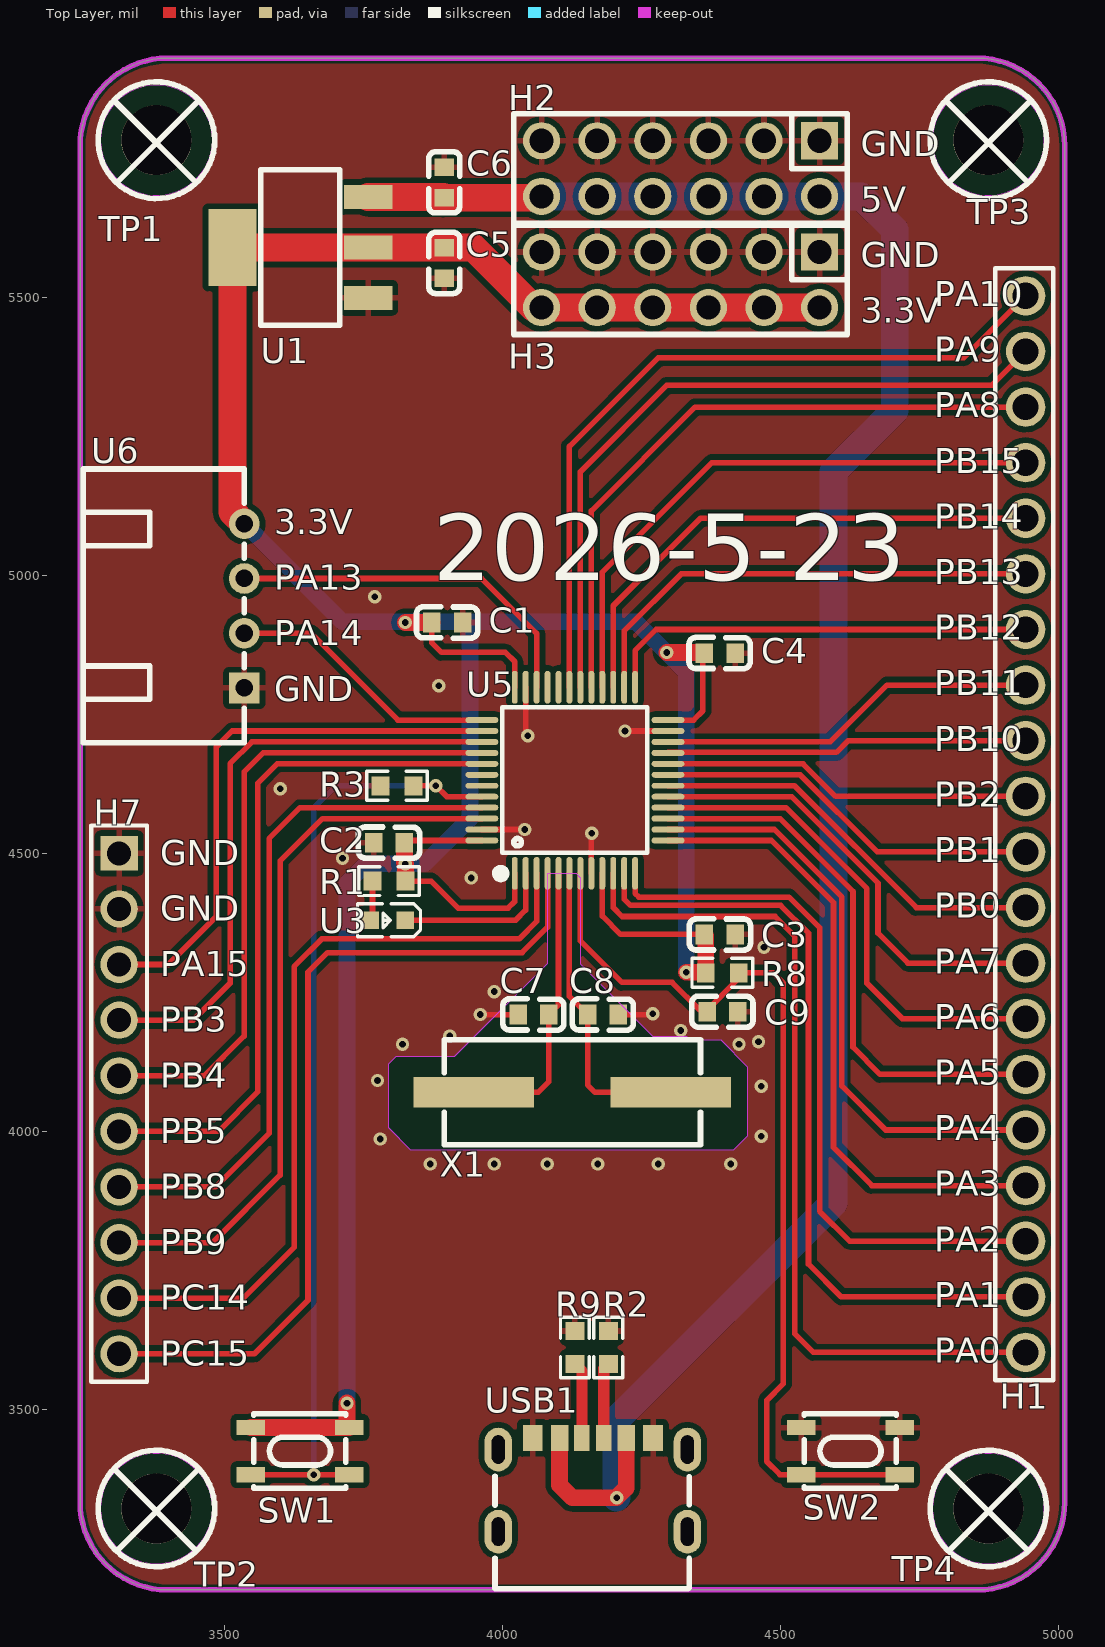
[diagram p0: Top Layer view]
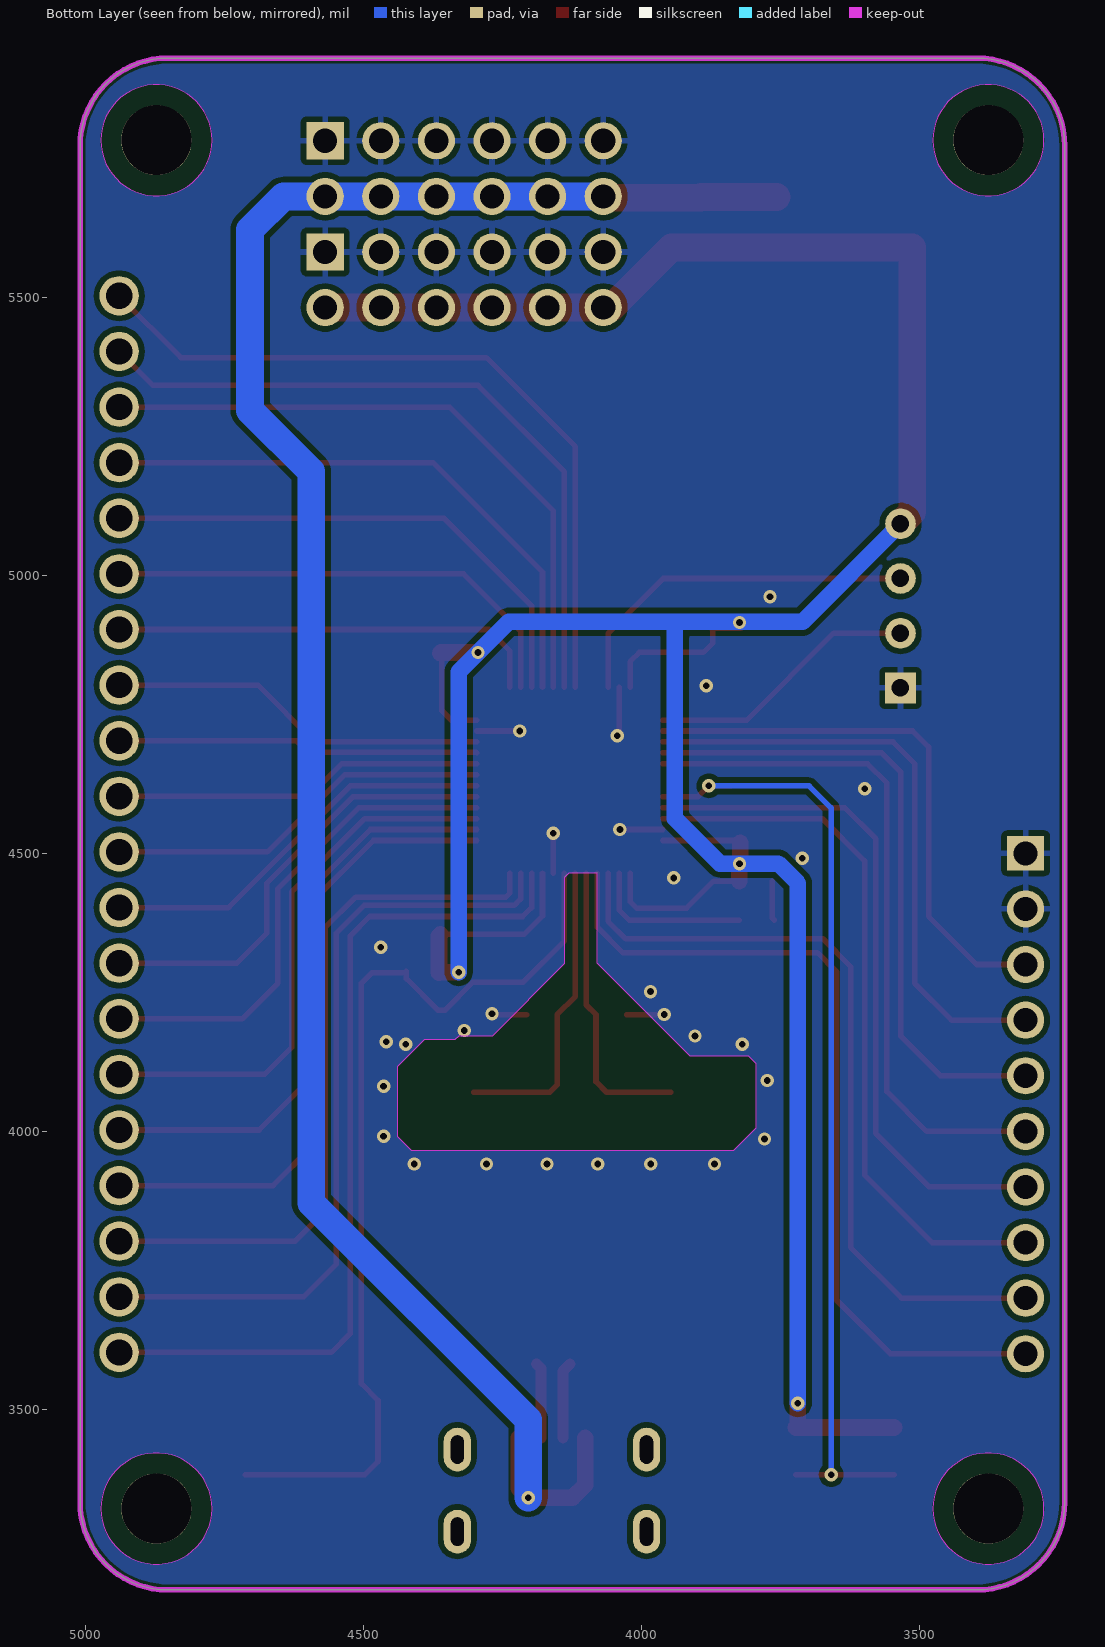
[diagram p1: Bottom Layer view, seen from below]
# Altium PCB MISC89146.pcbdoc
Units mil, origin at the board's own origin, x right, y up, seen from the top; angles counter-clockwise.
Board outline 1770.59 x 2754.61 mil, 2 copper layers (Top Layer, Bottom Layer), stack 62.206 mil thick; 30 components, 45 nets, 164 pads, 36 vias.

## Layer stack, top to bottom
Top Solder Mask Layer: solder mask 0.394, Dk 3.3
Top Layer: signal copper 1.379
Dielectric1: surface 59.449, FR4, Dk 4.5
Bottom Layer: signal copper 1.378
Bottom Solder Mask Layer: solder mask 0.394, Dk 3.3

## Board outline
3397.18,5930 ccw(c3397.18,5772.52) 3239.7,5772.52 3239.7,3332.87 ccw(c3397.18,3332.87) 3397.18,3175.39 4852.81,3175.39 ccw(c4852.81,3332.87) 5010.3,3332.87 5010.3,5772.52 ccw(c4852.81,5772.52) 4852.81,5930 3397.18,5930

## Design rules (kind name [scope] priority, off if disabled: settings)
BoardOutlineClearance copperThickness2oz_1 [All] p2 off: genericclearance=7.99 ignorepadtopadclearanceinfootprint=FALSE except(0: Arc-SplitContinuation Track-SplitContinuation SMDPad-SplitContinuation THPad-SplitContinuation Via-SplitContinuation Fill-SplitContinuation Region-SplitContinuation Poly-SplitContinuation Text-SplitContinuation Hole-SplitContinuation; 5.98: Arc-CutoutEdge SMDPad-CutoutEdge THPad-CutoutEdge Via-CutoutEdge Fill-CutoutEdge Region-CutoutEdge Text-CutoutEdge; 6.93: Hole-OutlineEdge Hole-CutoutEdge; 10: Poly-OutlineEdge Poly-CutoutEdge; 11.81: Arc-OutlineEdge Track-OutlineEdge SMDPad-OutlineEdge THPad-OutlineEdge Via-OutlineEdge Fill-OutlineEdge Region-OutlineEdge Text-OutlineEdge Track-CutoutEdge)
BoardOutlineClearance copperThickness1oz_1 [All] p4: genericclearance=4.02 ignorepadtopadclearanceinfootprint=FALSE except(0: Arc-SplitContinuation Track-SplitContinuation SMDPad-SplitContinuation THPad-SplitContinuation Via-SplitContinuation Fill-SplitContinuation Region-SplitContinuation Poly-SplitContinuation Text-SplitContinuation Hole-SplitContinuation; 6: SMDPad-CutoutEdge THPad-CutoutEdge Via-CutoutEdge Fill-CutoutEdge Region-CutoutEdge Text-CutoutEdge; 6.93: Hole-OutlineEdge Hole-CutoutEdge; 10: Poly-OutlineEdge Poly-CutoutEdge; 11.8: Arc-OutlineEdge Track-OutlineEdge SMDPad-OutlineEdge THPad-OutlineEdge Via-OutlineEdge Fill-OutlineEdge Region-OutlineEdge Text-OutlineEdge; 11.81: Arc-CutoutEdge Track-CutoutEdge)
Clearance copperThickness2oz [All] p1 off: gap=7.99 ignorepadtopadclearanceinfootprint=FALSE except(5.98: SMDPad-Track SMDPad-SMDPad THPad-Track SMDPad-THPad THPad-THPad Track-Via SMDPad-Via THPad-Via Via-Via Fill-Track Region-Track Fill-SMDPad Region-SMDPad Fill-THPad Region-THPad Fill-Via Region-Via Fill-Fill Fill-Region Region-Region Arc-Track Arc-SMDPad Arc-THPad Arc-Via Fill-Arc Region-Arc Arc-Arc Text-Track SMDPad-Text Text-THPad Text-Via Fill-Text Region-Text Arc-Text Text-Text; 6.93: Hole-Track Hole-SMDPad Hole-THPad Hole-Via Fill-Hole Region-Hole Hole-Arc Hole-Text; 10: Poly-Track Poly-SMDPad Poly-THPad Poly-Via Poly-Fill Poly-Region Poly-Poly Poly-Arc Poly-Text Poly-Hole)
Clearance copperThickness1oz [All] p3: gap=4.02 ignorepadtopadclearanceinfootprint=FALSE except(5.98: SMDPad-Track SMDPad-SMDPad THPad-Track SMDPad-THPad THPad-THPad Track-Via SMDPad-Via THPad-Via Via-Via Fill-Track Region-Track Fill-SMDPad Region-SMDPad Fill-THPad Region-THPad Fill-Via Region-Via Fill-Fill Fill-Region Region-Region; 6: Arc-Track Arc-SMDPad Arc-THPad Arc-Via Fill-Arc Region-Arc Arc-Arc Text-Track SMDPad-Text Text-THPad Text-Via Fill-Text Region-Text Arc-Text Text-Text; 6.93: Hole-Track Hole-SMDPad Hole-THPad Hole-Via Fill-Hole Region-Hole Hole-Arc Hole-Text; 10: Poly-Track Poly-SMDPad Poly-THPad Poly-Via Poly-Fill Poly-Region Poly-Poly Poly-Arc Poly-Text Poly-Hole)
Creepage creepage [All] p1: checkdistance=0 ignoreinternallayers=TRUE applytopolygonpour=TRUE
DiffPairsRouting differentialPair [All] p1: maxlimit=6 minlimit=6 mostfreqgap=6 toplayer_minwidth=5 toplayer_prefwidth=10 toplayer_maxwidth=100 toplayer_mingap=6 toplayer_prefgap=6 toplayer_maxgap=6 bottomlayer_minwidth=5 bottomlayer_prefwidth=10 bottomlayer_maxwidth=100 bottomlayer_mingap=6 bottomlayer_prefgap=6 bottomlayer_maxgap=6 maxuncoupledlength=10
HoleToHoleClearance otherClearance [All] p1: gap=11.81 allowstackedmicrovias=TRUE
Length netLength [All] p1: minlimit=0 maxlimit=0
MatchedLengths netLengthTolerance [All] p1: tolerance=1000
PasteMaskExpansion pasteMaskExpansion [All] p1: expansion=0
PlaneConnect innerPlane [All] p1: planeconnectstyle=Relief reliefexpansion=20 reliefentries=4 reliefconductorwidth=10 reliefairgap=10
PolygonConnect copperRegion [(InNet('GND'))] p1: connectstyle=Relief reliefconductorwidth=10 reliefentries=4 polygonreliefangle="90 Angle" airgapwidth=10 via.connectstyle=Relief via.reliefconductorwidth=10 via.reliefentries=4 via.polygonreliefangle="90 Angle" via.airgapwidth=10
RoutingVias viaSize [All] p1: holewidth=12.01 width=24.02 viastyle="Through Hole" minholewidth=11.81 minwidth=19.68 maxholewidth=248.03 maxwidth=393.7
SolderMaskExpansion solderMaskExpansion [IsVia] p1: expansion=-1000 istentingtop=TRUE
SolderMaskExpansion solderMaskExpansion [All] p2: expansion=2 istentingtop=FALSE
Width copperThickness2oz_2 [All] p1 off: maxlimit=100 minlimit=8 preferedwidth=10
Width copperThickness1oz_2 [All] p2: maxlimit=100 minlimit=5 preferedwidth=10

## Components (designator, comment, footprint, x,y, rotation, side; value= is the part's Value field where it differs from the comment)
C1 "100nF" C0603 3900,4915 r0 top
C2 "100nF" C0603 3795.45,4519.09 r0 top
C3 "100nF" C0603 4390,4354.09 r180 top
C4 "100nF" C0603 4390,4860 r0 top
C5 "2.2UF" C0603 3894.56,5561.33 r270 top
C6 "10UF" C0603 3894.56,5706.33 r270 top
C7 "22PF" C0603 4055,4210 r0 top
C8 "22PF" C0603 4180,4210 r0 top
C9 "1UF" C0603 4395,4215 r0 top
H1 "" HDR-TH_20P-P2.54-V-M-1 4940,4552.46 r90 top
H2 "" HDR-TH_12P-P2.54-V-M-R2-C6-S2.54 4319.56,5731.33 r180 top
H3 "" HDR-TH_12P-P2.54-V-M-R2-C6-S2.54 4319.56,5531.33 r180 top
H7 "" hdr-th_10p-p2.54-v-m-1 3310,4050 r270 top
R1 "1K" R0603 3795.15,4450 r180 top
R2 "5K1" R0603 4189.56,3611.33 r270 top
R3 "10K" R0603 3809.56,4621.33 r0 top
R8 "10K" R0603 4394.69,4285 r0 top
R9 "5K1" R0603 4129.56,3611.33 r270 top
SW1 "TS-KG89S-AT25F" SW-SMD_4P-L4.2-W3.3-P2.15-LS5.1 3635,3425 r180 top
SW2 "TS-KG89S-AT25F" SW-SMD_4P-L4.2-W3.3-P2.15-LS5.1 4625,3425 r180 top
TP1 "" M3 3376.97,5782.36 r0 top
TP2 "" M3 3376.97,3321.65 r0 top
TP3 "" M3 4873.03,5782.36 r0 top
TP4 "" M3 4873.03,3321.65 r0 top
U1 "" SOT_223 3634.7,5589.36 r90 top
U3 "LED_0603" LED_0603 3791.2,4379.5 r180 top
U5 "CH32V203C8T6" LQFP-48_L7.0-W7.0-P0.50-LS9.0-BL 4129.56,4631.33 r0 top
U6 "HCZZ0139-4" CONN-TH_4P-P2.50_HCZZ0139-4 3535,4945 r270 top
USB1 "" "USB_ TYPE-C-6P" 4156.74,3364.36 r0 top
X1 "8M-HC-49SMD" CRYSTAL-SMD_L11.4-W4.7-LS12.7 4125,4070 r180 top

## Footprints (in the part's own frame and the unit in brackets; to place one, negate y for a bottom-side part, rotate by r counter-clockwise, add the part's x,y. Pads: shape width x height; smd on the part's side, far side on the other; paste and mask are expansions set on the pad)
C0603 [mm]
  rect 0.8x0.9 smd paste+0 mask+0.051: 1(-0.7,0) 2(0.7,0)
  silkscreen extent -1.41,-0.71 1.39,0.72
CONN-TH_4P-P2.50_HCZZ0139-4 [mm]
  round 1.4 hole 0.8: 1(-3.75,0) 2(-1.25,0) 3(1.25,0)
  rect 1.4x1.4 hole 0.8: 4(3.75,0)
  silkscreen extent -6.25,-7.37 6.25,0
CRYSTAL-SMD_L11.4-W4.7-LS12.7 [mm]
  rect 5.5x1.4 smd paste+0 mask+0.051: 1(-4.5,0) 2(4.5,0)
  silkscreen extent -5.85,-2.4 5.85,2.4
hdr-th_10p-p2.54-v-m-1 [mm]
  rect 1.575x1.7 hole 1.1: 1(-11.43,0)
  round 1.7 hole 1.1: 2(-8.89,0) 3(-6.35,0) 4(-3.81,0) 5(-1.27,0) 6(1.27,0) 7(3.81,0) 8(6.35,0) 9(8.89,0) 10(11.43,0)
  silkscreen extent -12.7,-1.27 12.7,1.27
HDR-TH_12P-P2.54-V-M-R2-C6-S2.54 [mm]
  rect 1.7x1.7 hole 1.1: 1(-6.35,-1.27)
  round 1.7 hole 1.1: 2(-6.35,1.27) 3(-3.81,-1.27) 4(-3.81,1.27) 5(-1.27,-1.27) 6(-1.27,1.27) 7(1.27,-1.27) 8(1.27,1.27) 9(3.81,-1.27) 10(3.81,1.27) 11(6.35,-1.27) 12(6.35,1.27)
  silkscreen extent -7.62,-2.5 7.62,2.5
HDR-TH_20P-P2.54-V-M-1 [mm]
  round 1.8 hole 1.2 paste+0 mask+0.051: 1(-24.13,0) 2(-21.59,0) 3(-19.05,0) 4(-16.51,0) 5(-13.97,0) 6(-11.43,0) 7(-8.89,0) 8(-6.35,0) 9(-3.81,0) 10(-1.27,0) 11(1.27,0) 12(3.81,0) 13(6.35,0) 14(8.89,0) 15(11.43,0) 16(13.97,0) 17(16.51,0) 18(19.05,0) 19(21.59,0) 20(24.13,0)
  silkscreen extent -25.4,-1.27 25.4,1.4
LED_0603 [mil]
  rect 31.5x31.5 smd paste+0 mask+2: 1(-33.5,-0.4) 2(29.5,-0.2)
  silkscreen extent -61,-30 53,30
LQFP-48_L7.0-W7.0-P0.50-LS9.0-BL [mm]
  oval 0.27x1.5 smd paste+0 mask+0.05: 1(-2.75,-4.25) 2(-2.25,-4.25) 3(-1.75,-4.25) 4(-1.25,-4.25) 5(-0.75,-4.25) 6(-0.25,-4.25) 7(0.25,-4.25) 8(0.75,-4.25) 9(1.25,-4.25) 10(1.75,-4.25) 11(2.25,-4.25) 12(2.75,-4.25) 25(2.75,4.25) 26(2.25,4.25) 27(1.75,4.25) 28(1.25,4.25) 29(0.75,4.25) 30(0.25,4.25) 31(-0.25,4.25) 32(-0.75,4.25) 33(-1.25,4.25) 34(-1.75,4.25) 35(-2.25,4.25) 36(-2.75,4.25)
  oval 1.5x0.27 smd paste+0 mask+0.05: 13(4.25,-2.75) 14(4.25,-2.25) 15(4.25,-1.75) 16(4.25,-1.25) 17(4.25,-0.75) 18(4.25,-0.25) 19(4.25,0.25) 20(4.25,0.75) 21(4.25,1.25) 22(4.25,1.75) 23(4.25,2.25) 24(4.25,2.75) 37(-4.25,2.75) 38(-4.25,2.25) 39(-4.25,1.75) 40(-4.25,1.25) 41(-4.25,0.75) 42(-4.25,0.25) 43(-4.25,-0.25) 44(-4.25,-0.75) 45(-4.25,-1.25) 46(-4.25,-1.75) 47(-4.25,-2.25) 48(-4.25,-2.75)
  silkscreen extent -3.59,-4.46 3.3,3.34
M3 [mil]
  round 126 hole 126 paste+0 mask+4: 0(0,0)
  Board Outline Layer region: 100,0 90.1,-43.39 62.35,-78.18 22.25,-97.49 -22.25,-97.49 -62.35,-78.18 -90.1,-43.39 -100,0 -100,0 -90.1,43.39 -62.35,78.18 -22.25,97.49 22.25,97.49 62.35,78.18 90.1,43.39 100,0
  silkscreen extent -105,-105 105,105
R0603 [mil]
  rect 31.75x34.02 smd paste-3937.01 mask+2: 1(-29.66,0) 2(29.66,0)
  silkscreen extent -55,-26 55,26
SOT_223 [mil]
  rect 43.3x86.6 smd paste+0 mask+2: 1(-90.5,-123.05) 2(0,-123.05) 3(90.6,-123.05)
  rect 137.8x86.6 smd paste+0 mask+2: 4(0,120.95)
  silkscreen extent -140,-72 140,70
SW-SMD_4P-L4.2-W3.3-P2.15-LS5.1 [mm]
  rect 1.3x0.7 smd paste+0 mask+0.051: 1(-2.25,1.075) 2(2.25,1.075) 3(-2.25,-1.075) 4(2.25,-1.075)
  silkscreen extent -2.1,-1.7 2.1,1.7
"USB_ TYPE-C-6P" [mm]
  oval 1.25x2 hole 0.6 slot 1.3 at 90 deg paste+0 mask+0.05: 7(-4.193,1.611) 8(4.447,1.611) 9(-4.193,-2.139) 10(4.447,-2.139)
  rect 0.7x1.2 smd paste-100 mask+0.05: A5(-0.373,2.139) B5(0.627,2.139)
  rect 0.8x1.2 smd paste-100 mask+0.05: A9(1.647,2.139) B9(-1.393,2.139)
  rect 0.9x1.2 smd paste-100 mask+0.05: A12(2.877,2.139) B12(-2.623,2.139)
  silkscreen extent -4.34,-4.75 4.52,0.39

## Via types
v1: diameter 24.02, hole 12, Top Layer to Bottom Layer, 36 vias

## Nets (pads, with @x,y where several pads share a name; then routed paths per layer and width w, separated by ;. In a path a pad name is that pad's centre, name@x,y a point inside that pad or via, vN(x,y) a via of type N, cw(c..) or ccw(c..) an arc to the next point about the centre after c; other vN are vias at no path point)
3V: C1.1 C2.2 C3.2 C4.1 C5.1 H3.2 H3.4 H3.6 H3.8 H3.10 H3.12 R1.1 R8.1 SW1.3 SW1.4 U1.2 U1.4 U5.1 U5.9 U5.24 U5.36 U5.48 U6.1 | length 6231.4
  Top Layer w10: C2.2 3826.99,4523.06 U5.48 ; R1.1 3870.89,4450 3919.56,4401.33 4009.56,4401.33 4021.29,4413.06 U5.1 ; C1.1 3872.44,4878.45 3889.56,4861.33 4004.56,4861.33 4021.29,4844.6 U5.36 ; U5.9 4178.77,4387.12 4211.8,4354.09 C3.2 ; U5.24 4342.83,4739.6 4359.56,4756.33 4359.56,4857.12 C4.1
  Top Layer w30: SW1.4 SW1.3 3719.56,3471.35 v1(3719.56,3511.33) ; C2.2 3823.01,4482.88 v1(3824.56,4481.33) 3824.81,4481.08 R1.1 ; v1(3824.56,4915) C1.1 ; v1(4294.7,4861.19) 4361.25,4861.19 C4.1 ; v1(4329.56,4286.33) 4363.7,4286.33 R8.1 4365.03,4351.49 C3.2
  Top Layer w50: U6.1 3513.75,5113.89 U1.4 U1.2 3946.53,5589.36 4054.56,5481.33 H3.12 H3.10 H3.8 H3.6 H3.4 H3.2
  Bottom Layer w30: U6.1 3711.31,4916.33 3940.71,4916.33 ; v1(3719.56,3511.33) 3719.56,4446.33 3754.56,4481.33 v1(3824.56,4481.33) 3859.56,4481.33 3940.71,4562.49 3940.71,4916.33 ; v1(4329.56,4286.33) 4329.56,4826.33 v1(4294.7,4861.19) 4239.56,4916.33 3940.71,4916.33
$1N78: R9.2 USB1.A5 | length 138.3
  Top Layer w20: R9.2 4142.06,3569.16 USB1.A5
$1N90: R1.2 U3.2 | length 71.9
  Top Layer w10: U3.2 3765.49,4383.49 R1.2
$1N174: R2.2 USB1.B5 | length 136.5
  Top Layer w20: USB1.B5 4181.44,3573.55 R2.2
BOOT0: R3.2 SW1.1 SW1.2 U5.44 | length 1743.5
  Top Layer w10: SW1.2 v1(3659.66,3382.68) SW1.1 ; R3.2 v1(3879.56,4621.33) 3899.09,4601.8 U5.44
  Bottom Layer w10: v1(3659.66,3382.68) 3659.66,4581.44 3699.56,4621.33 v1(3879.56,4621.33)
GND: C1.2 C2.1 C3.1 C4.2 C5.2 C6.1 C7.1 C8.2 C9.2 H2.1 H2.3 H2.5 H2.7 H2.9 H2.11 H3.1 H3.3 H3.5 H3.7 H3.9 H3.11 H7.1 H7.2 R2.1 R3.1 R9.1 SW2.3 SW2.4 U1.1 U5.8 U5.23 U5.35 U5.47 U6.4 USB1.A12 USB1.B12 | length 446.4
  Top Layer w10: v1(3959.56,4210) C7.1 ; U5.47 v1(4039.56,4542.75) ; U5.35 4040.98,4714.91 v1(4044.56,4711.33) ; U5.8 4159.09,4535.86 v1(4159.56,4536.33) ; C8.2 4268.22,4210 v1(4269.56,4211.33) ; v1(4219.56,4719.91) U5.23
  other v1: 3869.56,3941.33 3984.36,3941.33 4079.57,3941.33 4170.76,3941.33 4279.56,3941.33 4409.46,3941.33 3779.56,3986.33 4464.56,3991.33 4464.56,4081.27 3774.56,4091.33 3819.56,4156.33 4424.56,4156.33 4459.56,4161.33 3904.56,4171.33 4319.56,4181.33 3984.56,4251.33 4469.56,4331.33 3942.87,4455.74 3711.64,4491.36 3599.56,4616.33 3884.56,4801.33 3769.56,4961.33
OSC-IN: C7.2 U5.5 X1.2 | length 524.6
  Top Layer w10: X1.2 4063.22,4070 4082.56,4089.34 C7.2 4100.03,4227.47 U5.5
OSC-OUT: C8.1 U5.6 X1.1 | length 549.4
  Top Layer w10: U5.6 4119.72,4242.72 C8.1 4152.44,4083.45 4165.89,4070 X1.1
PA0: H1.1 U5.10 | length 1553.3
  Top Layer w10: U5.10 4198.46,4402.43 4214.56,4386.33 4489.56,4386.33 4524.56,4351.33 4524.56,3636.33 4558.43,3602.46 H1.1
PA1: H1.2 U5.11 | length 1413
  Top Layer w10: U5.11 4218.14,4417.75 4229.56,4406.33 4499.56,4406.33 4549.56,4356.33 4549.56,3761.33 4608.43,3702.46 H1.2
PA2: H1.3 U5.12 | length 1296
  Top Layer w10: U5.12 4237.83,4428.06 4244.56,4421.33 4514.56,4421.33 4569.56,4366.33 4569.56,3856.33 4623.43,3802.46 H1.3
PA3: H1.4 U5.13 | length 1157.9
  Top Layer w10: U5.13 4482.83,4523.06 4594.56,4411.33 4594.56,3971.33 4663.43,3902.46 H1.4
PA4: H1.5 U5.14 | length 1066.1
  Top Layer w10: U5.14 4488.14,4542.75 4609.56,4421.33 4609.56,4081.33 4688.43,4002.46 H1.5
PA5: H1.6 U5.15 | length 997.7
  Top Layer w10: U5.15 4498.46,4562.43 4629.56,4431.33 4629.56,4151.33 4678.43,4102.46 H1.6
PA6: H1.7 U5.16 | length 900
  Top Layer w10: U5.16 4508.77,4582.12 4654.56,4436.33 4654.56,4266.33 4718.43,4202.46 H1.7
PA7: H1.8 U5.17 | length 819.8
  Top Layer w10: U5.17 4519.09,4601.8 4674.56,4446.33 4674.56,4356.33 4728.43,4302.46 H1.8
PA8: H1.18 U5.29 | length 1175.4
  Top Layer w10: U5.29 4159.09,5115.86 4345.68,5302.46 H1.18
PA9: H1.19 U5.30 | length 1277.7
  Top Layer w10: U5.30 4139.4,5186.17 4294.56,5341.33 4878.87,5341.33 H1.19
PA10: H1.20 U5.31 | length 1365.4
  Top Layer w10: U5.31 4119.72,5231.49 4279.56,5391.33 4828.87,5391.33 H1.20
PA11: U5.32
PA12: U5.33
PA13: U5.34 U6.2 | length 663.2
  Top Layer w10: U6.2 3961.68,4994.21 4060.66,4895.23 U5.34
PA14: U5.37 U6.3 | length 491.9
  Top Layer w10: U6.3 3655.1,4895.79 3811.29,4739.6 U5.37
PA15: H7.3 U5.38 | length 1004.8
  Top Layer w10: H7.3 3398.22,4300 3484.56,4386.33 3484.56,4691.33 3513.14,4719.91 U5.38
PB0: H1.9 U5.18 | length 733.9
  Top Layer w10: U5.18 4524.4,4621.49 4743.43,4402.46 H1.9
PB1: H1.10 U5.19 | length 700.6
  Top Layer w10: U5.19 4534.72,4641.17 4673.43,4502.46 H1.10
PB2: H1.11 U5.20 | length 667.3
  Top Layer w10: U5.20 4540.03,4660.86 4598.43,4602.46 H1.11
PB3: H7.4 U5.39 | length 1090.8
  Top Layer w10: H7.4 3443.22,4200 3509.56,4266.33 3509.56,4661.33 3548.46,4700.23 U5.39
PB4: H7.5 U5.40 | length 1171
  Top Layer w10: H7.5 3463.22,4100 3534.56,4171.33 3534.56,4646.33 3568.77,4680.54 U5.40
PB5: H7.6 U5.41 | length 1251.1
  Top Layer w10: H7.6 3488.22,4000 3559.56,4071.33 3559.56,4626.33 3594.09,4660.86 U5.41
PB6: U5.42
PB7: U5.43
PB8: H7.7 U5.45 | length 1245.2
  Top Layer w10: H7.7 3483.22,3900 3579.56,3996.33 3579.56,4526.33 3635.35,4582.12 U5.45
PB9: H7.8 U5.46 | length 1299
  Top Layer w10: H7.8 3478.22,3800 3599.56,3921.33 3599.56,4486.33 3675.66,4562.43 U5.46
PB10: H1.12 U5.21 | length 652.2
  Top Layer w10: U5.21 4297.67,4681.33 4599.56,4681.33 4620.68,4702.46 H1.12
PB11: H1.13 U5.22 | length 685.5
  Top Layer w10: U5.22 4588.46,4700.23 4690.68,4802.46 H1.13
PB12: H1.14 U5.25 | length 783.8
  Top Layer w10: U5.25 4237.83,4864.6 4275.68,4902.46 H1.14
PB13: H1.15 U5.26 | length 865.6
  Top Layer w10: U5.26 4218.14,4899.91 4320.68,5002.46 H1.15
PB14: H1.16 U5.27 | length 953.3
  Top Layer w10: U5.27 4198.46,4945.23 4355.68,5102.46 H1.16
PB15: H1.17 U5.28 | length 1049.7
  Top Layer w10: U5.28 4178.77,5005.54 4375.68,5202.46 H1.17
PC13: U3.1 U5.2 | length 289.9
  Top Layer w10: U3.1 4023.12,4379.9 4040.98,4397.75 U5.2
PC14: H7.9 U5.3 | length 1413.7
  Top Layer w10: H7.9 3533.22,3700 3624.56,3791.33 3624.56,4296.33 3674.56,4346.33 4029.56,4346.33 4060.66,4377.43 U5.3
PC15: H7.10 U5.4 | length 1530.6
  Top Layer w10: H7.10 3553.22,3600 3649.56,3696.33 3649.56,4286.33 3684.56,4321.33 4034.56,4321.33 4080.35,4367.12 U5.4
RST: C9.1 R8.2 SW2.1 SW2.2 U5.7 | length 1703.2
  Top Layer w10: U5.7 4139.4,4342.63 4214.3,4267.73 4304.3,4267.73 4354.3,4217.73 4366.74,4217.73 4423.65,4274.64 R8.2@4423.65,4287.73 ; R8.2 4485.89,4285 4504.56,4266.33 4504.56,3546.33 4474.56,3516.33 4474.56,3406.33 4498.21,3382.68 SW2.2 SW2.1
VBUS: C6.2 H2.2 H2.4 H2.6 H2.8 H2.10 H2.12 U1.3 USB1.A9 USB1.B9 | length 3771.2
  Top Layer w30: USB1.B9 4101.9,3363.98 4124.56,3341.33 v1(4204.56,3341.33) 4221.59,3358.36 USB1.A9
  Top Layer w50: U1.3 3893.37,5679.96 C6.2 4067,5678.77 H2.12
  Bottom Layer w50: H2.12 H2.10 H2.8 H2.6 H2.4 H2.2 4644.56,5681.33 4704.56,5621.33 4704.56,5296.33 4594.56,5186.33 4594.56,3871.33 4204.56,3481.33 v1(4204.56,3341.33)
pads on no net: TP1.0 TP2.0 TP3.0 TP4.0 USB1.7 USB1.8 USB1.9 USB1.10

## Polygon pours and split planes (outlines as drawn)
GND on Bottom Layer (solid, remove dead copper, pour order 2): 3000,6175 3000,3000 5265,3000 5265,6175
GND on Top Layer (solid, remove dead copper, pour order 0): 3000,6175 3000,3000 5265,3000 5265,6175

## Keep-outs
Board Outline Layer:
  region: 4080.35,4464.01 4131.88,4464.01 4139.56,4456.33 4139.56,4301.33 4269.56,4171.33 4329.29,4171.33 4336.14,4164.49 4391.4,4164.49 4439.56,4116.33 4439.56,3991.33 4414.56,3966.33 3834.56,3966.33 3794.56,4006.33 3794.56,4121.33 3808.18,4134.96 3913.18,4134.96 4080.35,4302.12
  lines w10: 3239.7,3332.87 3239.7,5772.52 cw(c3397.18,5772.52) 3397.18,5930 4852.81,5930 cw(c4852.81,5772.52) 5010.3,5772.52 5010.3,3332.87 cw(c4852.81,3332.87) 4852.81,3175.39 3397.18,3175.39 cw(c3397.18,3332.87) 3239.7,3332.87

## Silkscreen, mask and mechanical layers (free items; w line width, h text height)
Top Silkscreen Layer:
  text "GND" at 4643.56,5753.83 h45
  text "5V" at 4643.56,5653.83 h45
  text "GND" at 4643.56,5553.83 h45
  text "PA10" at 4775.71,5483.83 h45
  text "3.3V" at 4643.56,5453.83 h45
  text "PA9" at 4775.71,5383.83 h45
  text "PA8" at 4775.71,5283.83 h45
  text "PB15" at 4775.71,5183.83 h45
  text "PB14" at 4775.71,5083.83 h45
  text "3.3V" at 3588.91,5073.83 h45
  text "2026-5-23" at 3874.56,4991.33 h120
  text "PB13" at 4775.71,4983.83 h45
  text "PA13" at 3588.91,4973.83 h45
  text "PB12" at 4775.71,4883.83 h45
  text "PA14" at 3588.91,4873.83 h45
  text "PB11" at 4775.71,4783.83 h45
  text "GND" at 3588.91,4773.83 h45
  text "PB10" at 4775.71,4683.83 h45
  text "PB2" at 4775.71,4583.83 h45
  text "PB1" at 4775.71,4483.83 h45
  text "GND" at 3383.91,4478.83 h45
  text "PB0" at 4775.71,4383.83 h45
  text "GND" at 3383.91,4378.83 h45
  text "PA7" at 4775.71,4283.83 h45
  text "PA15" at 3383.91,4278.83 h45
  text "PA6" at 4775.71,4183.83 h45
  text "PB3" at 3383.91,4178.83 h45
  text "PA5" at 4775.71,4083.83 h45
  text "PB4" at 3383.91,4078.83 h45
  text "PA4" at 4775.71,3983.83 h45
  text "PB5" at 3383.91,3978.83 h45
  text "PA3" at 4775.71,3883.83 h45
  text "PB8" at 3383.91,3878.83 h45
  text "PA2" at 4775.71,3783.83 h45
  text "PB9" at 3383.91,3778.83 h45
  text "PA1" at 4775.71,3683.83 h45
  text "PC14" at 3383.91,3678.83 h45
  text "PA0" at 4775.71,3583.83 h45
  text "PC15" at 3383.91,3578.83 h45